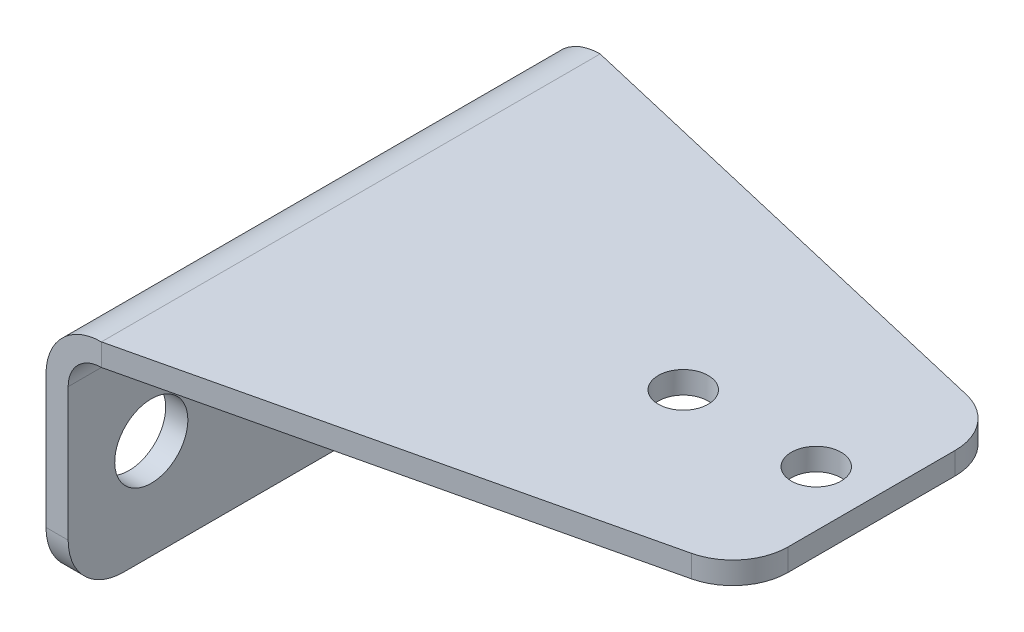
from build123d import *

# Parameters (mm, degrees)
BOSS_EXTRUDE1_DEPTH = 45
CUT_EXTRUDE1_REACH  = 72.774
SKETCH2_R           = 3.3
CUT_EXTRUDE2_REACH  = 74.201
SKETCH3_R           = 2.25
CUT_EXTRUDE3_REACH  = 74.201
FILLET1_R           = 5


with BuildPart() as part:
    # Sketch1 → Boss-Extrude1 (new body)
    with BuildSketch(Plane.XY):
        with BuildLine():
            Line((0, 0), (0, 17))
            ThreePointArc((0, 17), (1.464466094, 20.535533906), (5, 22))
            Line((5, 22), (52, 22))
            Line((52, 22), (52, 20))
            Line((52, 20), (5, 20))
            ThreePointArc((5, 20), (2.878679656, 19.121320344), (2, 17))
            Line((2, 17), (2, 0))
            Line((2, 0), (0, 0))
        make_face()
    extrude(amount=BOSS_EXTRUDE1_DEPTH)

    # Sketch2 → Cut-Extrude1 (cut, up to next)
    with BuildSketch(Plane(origin=(2, 0, 0), x_dir=(0, 0, -1), z_dir=(1, 0, 0)), mode=Mode.PRIVATE) as cut_extrude1_sk1:
        with Locations(Location((-37.5, 9, 0), (0, 0, 90))):
            Circle(SKETCH2_R)
    cut_extrude1_tool1 = extrude(cut_extrude1_sk1.sketch, amount=-CUT_EXTRUDE1_REACH, mode=Mode.PRIVATE) & part.part
    # Sketch2 → Cut-Extrude1 (cut, up to next)
    with BuildSketch(Plane(origin=(2, 0, 0), x_dir=(0, 0, -1), z_dir=(1, 0, 0)), mode=Mode.PRIVATE) as cut_extrude1_sk2:
        with Locations(Location((-7.5, 9, 0), (0, 0, 90))):
            Circle(SKETCH2_R)
    cut_extrude1_tool2 = extrude(cut_extrude1_sk2.sketch, amount=-CUT_EXTRUDE1_REACH, mode=Mode.PRIVATE) & part.part
    add(cut_extrude1_tool1.solids().sort_by_distance((2, 9, 37.5))[0], mode=Mode.SUBTRACT)
    add(cut_extrude1_tool2.solids().sort_by_distance((2, 9, 7.5))[0], mode=Mode.SUBTRACT)

    # Sketch3 → Cut-Extrude2 (cut, up to next)
    with BuildSketch(Plane(origin=(0, 22, 0), x_dir=(1, 0, 0), z_dir=(0, 1, 0)), mode=Mode.PRIVATE) as cut_extrude2_sk1:
        with Locations(Location((35, -22.5, 0), (0, 0, 270))):
            Circle(SKETCH3_R)
    cut_extrude2_tool1 = extrude(cut_extrude2_sk1.sketch, amount=-CUT_EXTRUDE2_REACH, mode=Mode.PRIVATE) & part.part
    # Sketch3 → Cut-Extrude2 (cut, up to next)
    with BuildSketch(Plane(origin=(0, 22, 0), x_dir=(1, 0, 0), z_dir=(0, 1, 0)), mode=Mode.PRIVATE) as cut_extrude2_sk2:
        with Locations(Location((47, -22.5, 0), (0, 0, 270))):
            Circle(SKETCH3_R)
    cut_extrude2_tool2 = extrude(cut_extrude2_sk2.sketch, amount=-CUT_EXTRUDE2_REACH, mode=Mode.PRIVATE) & part.part
    add(cut_extrude2_tool1.solids().sort_by_distance((35, 22, 22.5))[0], mode=Mode.SUBTRACT)
    add(cut_extrude2_tool2.solids().sort_by_distance((47, 22, 22.5))[0], mode=Mode.SUBTRACT)

    # Sketch4 → Cut-Extrude3 (cut, up to next)
    with BuildSketch(Plane(origin=(0, 22, 0), x_dir=(1, 0, 0), z_dir=(0, 1, 0)), mode=Mode.PRIVATE) as cut_extrude3_sk1:
        Polygon((5, 0), (52, -11), (52, 0), align=None)
    cut_extrude3_tool1 = extrude(cut_extrude3_sk1.sketch, amount=-CUT_EXTRUDE3_REACH, mode=Mode.PRIVATE) & part.part
    # Sketch4 → Cut-Extrude3 (cut, up to next)
    with BuildSketch(Plane(origin=(0, 22, 0), x_dir=(1, 0, 0), z_dir=(0, 1, 0)), mode=Mode.PRIVATE) as cut_extrude3_sk2:
        Polygon((5, -45), (52, -34), (52, -45), align=None)
    cut_extrude3_tool2 = extrude(cut_extrude3_sk2.sketch, amount=-CUT_EXTRUDE3_REACH, mode=Mode.PRIVATE) & part.part
    add(cut_extrude3_tool1.solids().sort_by_distance((36.333333, 22, 3.666667))[0], mode=Mode.SUBTRACT)
    add(cut_extrude3_tool2.solids().sort_by_distance((36.333333, 22, 41.333333))[0], mode=Mode.SUBTRACT)

    # Fillet1
    fillet1_edges = [part.edges().sort_by_distance(p)[0] for p in [
        (1, 0, 0),
        (1, 0, 45),
        (52, 21, 11),
        (52, 21, 34),
    ]]
    fillet(fillet1_edges, radius=FILLET1_R)


solid = part.part
